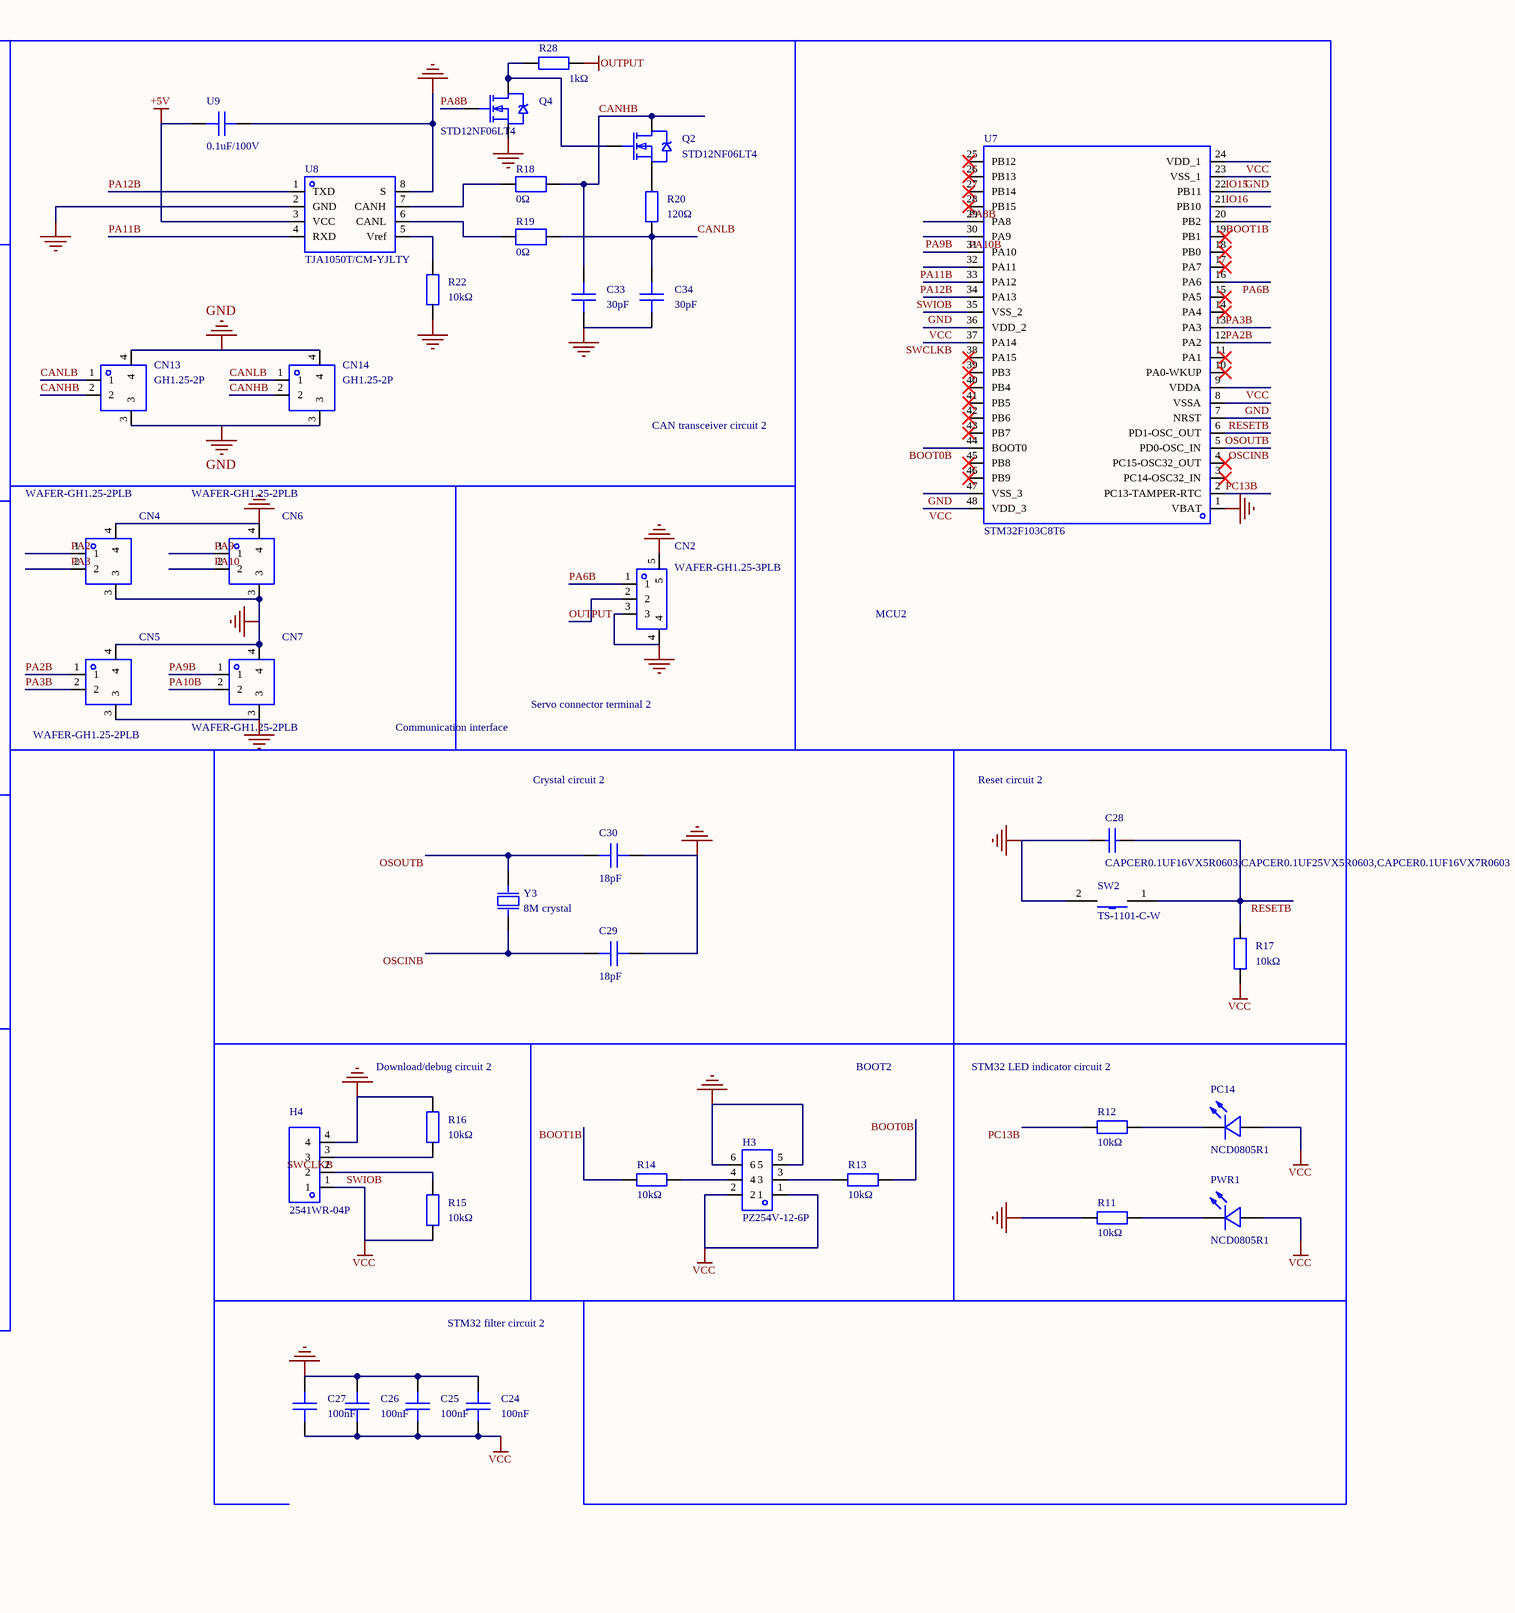
[diagram p0: MISC62500-4.schdoc, right]
# Altium project MISC62500-2.PrjPcb (part 2 of 2)
## Sheet MISC62500-4.schdoc (continued)
### Parts (continued)
Q2  STD12NF06LT4  [TO-252-3_L6.5-W5.8-P4.58-BL]
Q3  STD12NF06LT4  [TO-252-3_L6.5-W5.8-P4.58-BL]
Q4  STD12NF06LT4  [TO-252-3_L6.5-W5.8-P4.58-BL]
R1  10kΩ  [R0603]
R2  10kΩ  [R0603]
R3  10kΩ  [R0603]
R4  10kΩ  [R0603]
R5  10kΩ  [R0603]
R6  10kΩ  [R0603]
R7  10kΩ  [R0603]
R8  0Ω  [R0805]
R9  0Ω  [R0805]
R10  120Ω  [R0805]
R11  10kΩ  [R0603]
R12  10kΩ  [R0603]
R13  10kΩ  [R0603]
R14  10kΩ  [R0603]
R15  10kΩ  [R0603]
R16  10kΩ  [R0603]
R17  10kΩ  [R0603]
R18  0Ω  [R0805]
R19  0Ω  [R0805]
R20  120Ω  [R0805]
R21  10kΩ  [R0603]
R22  10kΩ  [R0603]
R27  1kΩ  [R0805]
R28  1kΩ  [R0805]
SW1  TS-1101-C-W  [SW-SMD_L6.0-W3.3-LS8.0]
SW2  TS-1101-C-W  [SW-SMD_L6.0-W3.3-LS8.0]
SW5  SK12D07VG4  [SW-TH_SK12D07VG4]
U1  STM32F103C8T6  [LQFP-48_L7.0-W7.0-P0.50-LS9.0-BL]
U2  0.1uF/100V  [C0805]
U3  AMS1117-5.0  [SOT-89-3_L4.5-W2.5-P1.50-LS4.2-BR]
U4  TJA1050T/CM-YJLTY  [SOIC-8_L4.9-W3.9-P1.27-LS6.0-BL]
U6  XT30U-F  [CONN-TH_XT30U-F]
U7  STM32F103C8T6  [LQFP-48_L7.0-W7.0-P0.50-LS9.0-BL]
U8  TJA1050T/CM-YJLTY  [SOIC-8_L4.9-W3.9-P1.27-LS6.0-BL]
U9  0.1uF/100V  [C0805]
Y2  8M crystal  [HC-49S_L11.5-W4.7-P4.88]
Y3  8M crystal  [HC-49S_L11.5-W4.7-P4.88]

### Blocks framed on the sheet
STM32 power circuit: C1-C4 LDO1
STM32 filter circuit: C5-C8
CAN transceiver circuit 2: C33 C34 CN13 CN14 Q2 Q4 R18-R20 R22 R28 U8 U9
MCU2: U7
STM32 LED indicator circuit: PC13 PWR R1 R2
Download/debug circuit: H2 R5 R6
Reset circuit: C9 R7 SW1
Communication interface: CN4-CN7
Servo connector terminal 2: CN2
Crystal circuit 2: C29 C30 Y3
Reset circuit 2: C28 R17 SW2
MCU: U1
Servo connector terminal: CN1
Voltage regulator module: C14-C17 U3
Download/debug circuit 2: H4 R15 R16
BOOT2: H3 R13 R14
STM32 LED indicator circuit 2: PC14 PWR1 R11 R12
CAN transceiver circuit: C18 C19 CN11 CN12 Q1 Q3 R8-R10 R21 R27 U2 U4

### Nets
+5V: C1.2 C2.2 C15.1 C17.1 LDO1.1(VIN) LDO1.3(CE) U2.1 U3.2(VOUT) U4.3(VCC) U8.3(VCC) U9.1
GND: C1.1 C2.1 C3.1 C4.1 C5.1 C6.1 C7.1 C8.1 C9.1 C10.2 C11.2 C14.1 C15.2 C16.1 C17.2 C18.1 C19.1 C24.1 C25.1 C26.1 C27.1 C28.1 C29.2 C30.2 C33.1 C34.1 CN1.3 CN1.4 CN1.5 CN2.3 CN2.4 CN2.5 CN3.1 CN3.2 CN4.3 CN4.4 CN5.3 CN5.4 CN6.3 CN6.4 CN7.3 CN7.4 CN10.1 CN10.2 CN11.3 CN11.4 CN12.3 CN12.4 CN13.3 CN13.4 CN14.3 CN14.4 H1.5 H1.6 H2.4 H3.5 H3.6 H4.4 LDO1.2(VSS) Q3.3(S) Q4.3(S) R1.2 R6.1 R11.2 R16.1 R21.1 R22.1 SW1.2 SW2.2 SW5.4 SW5.5 U1.1(VBAT) U1.8(VSSA) U1.23(VSS_1) U1.35(VSS_2) U1.47(VSS_3) U2.2 U3.1(ADJ/GND) U4.2(GND) U4.8(S) U6.1(-) U7.1(VBAT) U7.8(VSSA) U7.23(VSS_1) U7.35(VSS_2) U7.47(VSS_3) U8.2(GND) U8.8(S) U9.2
OUTPUT: C14.2 C16.2 CN1.2 CN2.2 R27.2 R28.2 SW5.2 U3.3(VIN)
VCC: C3.2 C4.2 C5.2 C6.2 C7.2 C8.2 C24.2 C25.2 C26.2 C27.2 H1.1 H1.2 H2.1 H3.1 H3.2 H4.1 LDO1.5(VOUT) PC13.1(+) PC14.1(+) PWR.1(+) PWR1.1(+) R5.2 R7.2 R15.2 R17.2 U1.9(VDDA) U1.24(VDD_1) U1.36(VDD_2) U1.48(VDD_3) U7.9(VDDA) U7.24(VDD_1) U7.36(VDD_2) U7.48(VDD_3)
BOOT0: R3.1 U1.44(BOOT0)
BOOT0B: R13.1 U7.44(BOOT0)
BOOT1: R4.2 U1.20(PB2)
BOOT1B: R14.2 U7.20(PB2)
CANH: C18.2 CN11.2 CN12.2 Q1.2(D) R8.2
CANHB: C33.2 CN13.2 CN14.2 Q2.2(D) R18.2
CANL: C19.2 CN11.1 CN12.1 R9.2 R10.1
CANLB: C34.2 CN13.1 CN14.1 R19.2 R20.1
IO4: U1.22(PB11)
IO5: U1.21(PB10)
IO15: U7.22(PB11)
IO16: U7.21(PB10)
OSCIN: C10.1 U1.5(PD0-OSC_IN) Y2.1(OSC1)
OSCINB: C29.1 U7.5(PD0-OSC_IN) Y3.1(OSC1)
OSOUT: C11.1 U1.6(PD1-OSC_OUT) Y2.2(OSC2)
OSOUTB: C30.1 U7.6(PD1-OSC_OUT) Y3.2(OSC2)
PA2: CN4.1 U1.12(PA2)
PA2B: CN5.1 U7.12(PA2)
PA3: CN4.2 U1.13(PA3)
PA3B: CN5.2 U7.13(PA3)
PA6: CN1.1 U1.16(PA6)
PA6B: CN2.1 U7.16(PA6)
PA8: Q3.1(G) U1.29(PA8)
PA8B: Q4.1(G) U7.29(PA8)
PA9: CN6.1 U1.30(PA9)
PA9B: CN7.1 U7.30(PA9)
PA10: CN6.2 U1.31(PA10)
PA10B: CN7.2 U7.31(PA10)
PA11: U1.32(PA11) U4.4(RXD)
PA11B: U7.32(PA11) U8.4(RXD)
PA12: U1.33(PA12) U4.1(TXD)
PA12B: U7.33(PA12) U8.1(TXD)
PC13: R2.2 U1.2(PC13-TAMPER-RTC)
PC13B: R12.2 U7.2(PC13-TAMPER-RTC)
POWER: SW5.1 U6.2(+)
RESET: C9.2 R7.1 SW1.1 U1.7(NRST)
RESETB: C28.2 R17.1 SW2.1 U7.7(NRST)
SWCLK: H2.3 R6.2 U1.37(PA14)
SWCLKB: H4.3 R16.2 U7.37(PA14)
SWIO: H2.2 R5.1 U1.34(PA13)
SWIOB: H4.2 R15.1 U7.34(PA13)
NetH1_3: H1.3 R3.2
NetH1_4: H1.4 R4.1
NetH3_3: H3.3 R13.2
NetH3_4: H3.4 R14.1
NetPC13_2: PC13.2(-) R2.1
NetPC14_2: PC14.2(-) R12.1
NetPWR1_2: PWR1.2(-) R11.1
NetPWR_2: PWR.2(-) R1.1
NetQ1_1: Q1.1(G) Q3.2(D) R27.1
NetQ1_3: Q1.3(S) R10.2
NetQ2_1: Q2.1(G) Q4.2(D) R28.1
NetQ2_3: Q2.3(S) R20.2
NetR8_1: R8.1 U4.7(CANH)
NetR9_1: R9.1 U4.6(CANL)
NetR18_1: R18.1 U8.7(CANH)
NetR19_1: R19.1 U8.6(CANL)
NetR21_2: R21.2 U4.5(Vref)
NetR22_2: R22.2 U8.5(Vref)

Not connected (* = marked no-connect by the designer): LDO1 4(NC)*; SW5 3*; U1 3(PC14-OSC32_IN)* 4(PC15-OSC32_OUT)* 10(PA0-WKUP)* 11(PA1)* 14(PA4)* 15(PA5)* 17(PA7)* 18(PB0)* 19(PB1)* 25(PB12)* 26(PB13)* 27(PB14)* 28(PB15)* 38(PA15)* 39(PB3)* 40(PB4)* 41(PB5)* 42(PB6)* 43(PB7)* 45(PB8)* 46(PB9)*; U7 3(PC14-OSC32_IN)* 4(PC15-OSC32_OUT)* 10(PA0-WKUP)* 11(PA1)* 14(PA4)* 15(PA5)* 17(PA7)* 18(PB0)* 19(PB1)* 25(PB12)* 26(PB13)* 27(PB14)* 28(PB15)* 38(PA15)* 39(PB3)* 40(PB4)* 41(PB5)* 42(PB6)* 43(PB7)* 45(PB8)* 46(PB9)*

### Notes on the sheet
- BOOT
- Crystal circuit
- (near SW5) Power switch
- STM32 filter circuit 2
- 2026-05-12
- Schematic
- Sheet
- Item code
- Reviewed
- Drawn
- Revision
- Size
- page
- Total
- A4
- 1
- 2

### Library data of the parts
C1 C4 C9 C28 = CAPCER0.1UF16VX5R0603,CAPCER0.1UF25VX5R0603,CAPCER0.1UF16VX7R0603: AddInBom: yes; ModelId: ac125912035d415993ca9572d50418b1; ModelName: C0603_L1.6-W0.8-H0.8; ModelTransform: 62.992,31.496,0,0,0,0,0,0,0; Symbol: CAPCER0.1UF16VX5R0603,CAPCER0.1UF25VX5R0603,CAPCER0.1UF16VX7R0603; Device: CAPCER0.1UF16VX5R0603,CAPCER0.1UF25VX5R0603,CAPCER0.1UF16VX7R0603; LCSC Part Name: CAPCER0.1UF16VX5R0603,CAPCER0.1UF25VX5R0603,CAPCER0.1UF16VX7R0603; SupplierPart: C9900012833; ManufacturerPart: CAPCER0.1UF16VX5R0603,CAPCER0.1UF25VX5R0603,CAPCER0.1UF16VX7R0603; Supplier Footprint: C0603; JLCPCB Part Class: Extended Part; Supplier: LCSC; ConvertToPcb: yes; FootprintName: C0603
C2 C3 = GRM188R71C105KE15D: Capacitance: 1uF; Tolerance: ±10%; Rated voltage: 16V; Dielectric (temp coefficient): X7R;; Manufacturer: muRata(村田); AddInBom: yes; ModelId: ac125912035d415993ca9572d50418b1; ModelName: C0603_L1.6-W0.8-H0.8; ModelTransform: 62.992,31.496,0,0,0,0,0,0,0; Symbol: GRM188R71C105KE15D; Device: GRM188R71C105KE15D; LCSC Part Name: 1uF ±10% 16V; SupplierPart: C77049; ManufacturerPart: GRM188R71C105KE15D; Supplier Footprint: 0603; JLCPCB Part Class: Extended Part; Datasheet: example.com/upload/public/pdf/source/20200305/C490387_23319AE8C154DEB24C505E6C82A8106A.pdf; Supplier: LCSC; ConvertToPcb: yes; FootprintName: C0603; Value: 1uF; Voltage Rated: 16V; Temperature Coefficient: X7R
C5-C8 C14 C15 C24-C27 = C1608X7S2A104K080AE: Capacitance: 100nF; Tolerance: ±10%; Rated voltage: 100V; Dielectric (temp coefficient): X7S;; Manufacturer: TDK; AddInBom: yes; ModelId: ac125912035d415993ca9572d50418b1; ModelName: C0603_L1.6-W0.8-H0.8; ModelTransform: 62.992,31.496,0,0,0,0,0,0,0; Symbol: C1608X7S2A104K080AE; Device: C1608X7S2A104K080AE; LCSC Part Name: 100nF ±10% 100V; SupplierPart: C3840667; ManufacturerPart: C1608X7S2A104K080AE; Supplier Footprint: 0603; JLCPCB Part Class: Extended Part; Datasheet: example.com/upload/public/pdf/source/20230606/B9E1D4FA5049A6C4984F2DC41D008D88.pdf; Supplier: LCSC; ConvertToPcb: yes; FootprintName: C0603; Value: 100nF; Voltage Rated: 100V; Temperature Coefficient: X7S
C10 C11 C29 C30 = C1608C0G1H180J080AA: Capacitance: 18pF; Tolerance: ±5%; Rated voltage: 50V; Dielectric (temp coefficient): C0G;; Manufacturer: TDK; AddInBom: yes; ModelId: ac125912035d415993ca9572d50418b1; ModelName: C0603_L1.6-W0.8-H0.8; ModelTransform: 62.992,31.496,0,0,0,0,0,0,0; Symbol: C1608C0G1H180J080AA; Device: C1608C0G1H180J080AA; LCSC Part Name: 18pF ±5% 50V; SupplierPart: C3902597; ManufacturerPart: C1608C0G1H180J080AA; Supplier Footprint: 0603; JLCPCB Part Class: Extended Part; Datasheet: example.com/upload/public/pdf/source/20230606/A83975C7E70EF5AFCD4A17254ABD78F2.pdf; Supplier: LCSC; ConvertToPcb: yes; FootprintName: C0603; Value: 18pF; Voltage Rated: 50V; Temperature Coefficient: C0G
C16 = CL10A106KP8NNNC: Capacitance: 10uF; Tolerance: ±10%; Rated voltage: 10V; Dielectric (temp coefficient): X5R;; Manufacturer: SAMSUNG(三星); AddInBom: yes; ModelId: ac125912035d415993ca9572d50418b1; ModelName: C0603_L1.6-W0.8-H0.8; ModelTransform: 62.992,31.496,0,0,0,0,0,0,0; Symbol: CL10A106KP8NNNC; Device: CL10A106KP8NNNC; LCSC Part Name: 10uF ±10% 10V; SupplierPart: C19702; ManufacturerPart: CL10A106KP8NNNC; Supplier Footprint: 0603; JLCPCB Part Class: Basic Part; Datasheet: example.com/upload/public/pdf/source/20160218/1457707763339.pdf; Supplier: LCSC; ConvertToPcb: yes; FootprintName: C0603; Value: 10uF; Voltage Rated: 10V; Temperature Coefficient: X5R
C17 = CL10A226MQ8NRNC: Capacitance: 22uF; Tolerance: ±20%; Rated voltage: 6.3V; Dielectric (temp coefficient): X5R;; Manufacturer: SAMSUNG(三星); AddInBom: yes; ModelId: ac125912035d415993ca9572d50418b1; ModelName: C0603_L1.6-W0.8-H0.8; ModelTransform: 62.992,31.496,0,0,0,0,0,0,0; Symbol: CL10A226MQ8NRNC; Device: CL10A226MQ8NRNC; LCSC Part Name: 22uF ±20% 6.3V; SupplierPart: C59461; ManufacturerPart: CL10A226MQ8NRNC; Supplier Footprint: 0603; JLCPCB Part Class: Basic Part; Datasheet: example.com/upload/public/pdf/source/20160218/1457707763339.pdf; Supplier: LCSC; ConvertToPcb: yes; FootprintName: C0603; Value: 22uF; Voltage Rated: 6.3V; Temperature Coefficient: X5R
C18 C19 C33 C34 = 0805N300J500CT: Capacitance: 30pF; Tolerance: ±5%; Rated voltage: 50V; Dielectric (temp coefficient): NP0;; Manufacturer: Walsin(华新科); AddInBom: yes; ModelId: 1ba041120af144c991958decab20d241; ModelName: C0805_L2.0-W1.3-H1.3; ModelTransform: 78.74,51.181,0,0,0,0,0,0.0005,0; Symbol: 0805N300J500CT; Device: 0805N300J500CT; LCSC Part Name: 30pF ±5% 50V; SupplierPart: C296096; ManufacturerPart: 0805N300J500CT; Supplier Footprint: 0805; JLCPCB Part Class: Extended Part; Datasheet: example.com/upload/public/pdf/source/20190509/C384834_C04286DA86A56A9914642D37A195BF18.pdf; Supplier: LCSC; ConvertToPcb: yes; FootprintName: C0805; Value: 30pF; Voltage Rated: 50V; Temperature Coefficient: NP0
CN1 CN2 = WAFER-GH1.25-3PLB: 插针结构:1x3P;间距:1.25mm;安装方式:立贴;参考系列:GH;总PIN数:3P;排数:1;每排PIN数:3;额定电流:1A;工作温度范围:-25℃~+85℃;; Manufacturer: XUNPU(讯普); AddInBom: yes; ModelId: 4873dadba1a240aabfda9d65a8d79f0f; ModelTransform: 277.9522,194.882,0,0,0,0,0,-21.89,0; Pins Structure: 1x3P; Pitch: 1.25mm; Reference Series: GH; Number of PINs Per Row: 3; Current Rating (Max): 1A; Symbol: WAFER-GH1.25-3PLB; Device: WAFER-GH1.25-3PLB; LCSC Part Name: 1x3P 间距:1.25mm 立贴 系列:GH; SupplierPart: C3029369; ManufacturerPart: WAFER-GH1.25-3PLB; Supplier Footprint: SMD,P=1.25mm; JLCPCB Part Class: Extended Part; Datasheet: example.com/upload/public/pdf/source/20220527/44F824AAC8C2B617205E15955FF9C23D.pdf; Supplier: LCSC; ConvertToPcb: yes; FootprintName: CONN-SMD_3P-P1.25_XUNPU_WAFER-GH1.25-3PLB; ModelName: CONN-SMD_3P-P1.25_XUNPU_WAFER-GH1.25-3PLB; Mounting Style: Vertical SMD; Number of Pins: 3P; Number of Rows: 1; Operating Temperature Range: -25℃~+85℃
CN3 CN10 = 2060-451/998-404: 结构:1x1P;间距:-;颜色:白色;安装方式:-;总PIN数:1P;每排PIN数:1;排数:1;额定电流:9A;额定电压:600V;线规 - AWG:18~24;线规 - 平方毫米:-;工作温度:-60℃~+105℃;; Manufacturer: WAGO(万可); AddInBom: yes; ModelId: 2b3842d5616144ad98afb9a8d8e70ac0; ModelTransform: 515.747,153.543,0,0,0,0,-20.512,0,0; Number of Positions or Pins: 1x1P; Number of PINs Per Row: 1; Current Rating: 9A; Voltage Rating (Max): 600V; Wire Gauge - AWG: 18~24; Symbol: 2060-451/998-404; Device: 2060-451/998-404; LCSC Part Name: 1x1P 每排P数:1 排数:1; SupplierPart: C2765054; ManufacturerPart: 2060-451/998-404; Supplier Footprint: SMD,P=4mm; JLCPCB Part Class: Extended Part; Datasheet: example.com/upload/public/pdf/source/20210406/C2765054_9C4366D01569C61DE4D9DE6FC53C47DE.pdf; Supplier: LCSC; ConvertToPcb: yes; FootprintName: CONN-SMD_L12.7-W3.9_2060-451-998-404; ModelName: CONN-SMD_L12.7-W3.9_2060-451-998-404; Pitch: -; Color: White; Mounting Type: -; Number of Pins: 1P; Number of Rows: 1; Wire Gauge - mm2: -; Operating Temperature: -60℃~+105℃
CN4-CN7 CN11-CN14 = WAFER-GH1.25-2PLB: 插针结构:1x2P;间距:1.25mm;安装方式:立贴;参考系列:GH;总PIN数:2P;排数:1;每排PIN数:2;行距:-;额定电流:1A;触头材质:黄铜;触头镀层:-;工作温度范围:-25℃~+85℃;; Manufacturer: XUNPU(讯普); AddInBom: yes; ModelId: 0c15e313285a4ca08f633459465ca938; ModelTransform: 226.7712,194.8815,0,180,0,0,0,-11.968,0; Pins Structure: 1x2P; Pitch: 1.25mm; Reference Series: GH; Number of PINs Per Row: 2; Current Rating: 1A; Voltage Rating: 125V; Plastic Material: LCP; Supplementary Features: Auxiliary solder pad; Z-Height of the Board: 4.2mm; X-Length of Bottom Edge on Board (Spacing Line): 5.75mm; Y-Width of Bottom Edge on Board: 4.95mm; Symbol: WAFER-GH1.25-2PLB; Device: WAFER-GH1.25-2PLB; LCSC Part Name: 1x2P 间距:1.25mm 立贴 系列:GH; SupplierPart: C3029368; Supplier Footprint: SMD,P=1.25mm; JLCPCB Part Class: Extended Part; Datasheet: example.com/upload/public/pdf/source/20220527/44F824AAC8C2B617205E15955FF9C23D.pdf; Supplier: LCSC; ConvertToPcb: yes; FootprintName: CONN-TH_2P-P1.25_XUNPU_WAFER-GH1.25-2PLB; ModelName: CONN-TH_2P-P1.25_XUNPU_WAFER-GH1.25-2PLB; Mounting Type: Vertical SMD; Number of Pins: 2P; Number of Rows: 1; Row Spacing: -; Contact Material: Brass; Contact Plating: -; Operating Temperature: -25℃~+85℃; Flame Retardant Rating: -; Color: Beige
  CN4-CN7: ManufacturerPart: WAFER-GH1.25-2PLB
  CN11-CN14: Manufacturer Part: GH1.25-2P
H1 H3 = PZ254V-12-6P: 插针结构:2x3P;间距:2.54mm;行距:2.54mm;圆针/方针:方针;安装类型:直插;排数:双排;总PIN位数:6P;额定电流:-;额定电压:-;配合针长度:6mm;塑高:2.5mm;端接针长度:3mm;触头材质:黄铜;触头镀层:-;工作温度范围:-40℃~+105℃;颜色:黑色;; Manufacturer: XFCN(兴飞); AddInBom: yes; ModelId: 6bc2347a11144808b30843246bd74e32; ModelTransform: 299.9994,200,0,0,0,0,0,0,-118.11; Pin Structure: 2x3P; Pitch: 2.54mm; Circluar Pins/Square Pins: Square pin; Symbol: PZ254V-12-6P; Device: PZ254V-12-6P; LCSC Part Name: 间距:2.54mm 2x3P 直插 方针; SupplierPart: C492420; ManufacturerPart: PZ254V-12-6P; Supplier Footprint: 插件,P=2.54mm; JLCPCB Part Class: Extended Part; Datasheet: example.com/upload/public/pdf/source/20200309/C492420_BAECB307B001054C09D200388220EAE6.pdf; Supplier: LCSC; ConvertToPcb: yes; FootprintName: HDR-TH_6P-P2.54-V-M-R2-C3-S2.54; ModelName: HDR-TH_6P-P2.54-V-M-R2-C3-S2.54; Row Spacing: 2.54mm; Mounting Type: Through-hole; Number of Rows: Dual row; Number of Pins: 6P; Current Rating (Max): -; Voltage Rating (Max): -; Length of Mating Pin: 6mm; Insulation Height: 2.5mm; Length of End Connection Pin: 3mm; Contact Material: Brass; Contact Plating: -; Operating Temperature Range: -40℃~+105℃; Color: Black
H2 H4 = 2541WR-04P: Pitch: 2.54mm; Mounting: right-angle THT; Rows: single; Mating pin length: 6mm; Plastic height: 2.54mm;; Manufacturer: HanElectricity(瀚源); AddInBom: yes; ModelId: 91498ce4cc554a519d8986aa62dd6bb1; ModelTransform: 399.999,405.511,0,0,0,0,0,-188.976,-118.11; Symbol: 2541WR-04P; Device: 2541WR-04P; LCSC Part Name: 间距:2.54mm 弯插; SupplierPart: C5383097; ManufacturerPart: 2541WR-04P; Supplier Footprint: 弯插,P=2.54mm; JLCPCB Part Class: Extended Part; Datasheet: example.com/upload/public/pdf/source/20230410/E05CF6F056E300DA9C417F17E461DF93.pdf; Supplier: LCSC; ConvertToPcb: yes; FootprintName: HDR-TH_4P-P2.54-H-M-W10.4-N; ModelName: HDR-TH_4P-P2.54-H-M-W10.4-N; Mounting Type: Right-angle THT; Number of Rows: Single row; Length of Mating Pin: 6mm; Insulation Height: 2.54mm
LDO1 = ME6211C33M5G-N: Output type: fixed; Max input voltage: 6V; Output voltage: 3.3V; Max output current: 500mA; PSRR: 70dB; Output polarity: positive;; Manufacturer: MICRONE(南京微盟); AddInBom: yes; ModelId: 0a2a1b8f50944f73965918ad6e5fe167; ModelName: SOT-23-5_L2.9-W1.6-H1.1-LS2.8-P0.95; ModelTransform: 118.60433,114.173,0,90,0,0,0.0005,0.0005,0; Dropout Voltage: 260mV@(200mA); Number of Outputs: 1; Symbol: ME6211C33M5G-N; Device: ME6211C33M5G-N; LCSC Part Name: 输入6V 输出3.3V 500mA; SupplierPart: C82942; ManufacturerPart: ME6211C33M5G-N; Supplier Footprint: SOT-23-5; JLCPCB Part Class: Extended Part; Datasheet: example.com/upload/public/pdf/source/20170918/C82942_1505727073070976520.pdf; Supplier: LCSC; ConvertToPcb: yes; FootprintName: SOT-23-5_L3.0-W1.7-P0.95-LS2.8-BL; Output Type: Fixed; Maximum Input Voltage: 6V; Output Voltage: 3.3V; MAX Output Current: 500mA; Power Supply Rejection Ratio (PSRR): 70dB; Output Polarity: Positive
PC13 PC14 PWR PWR1 = NCD0805R1: 灯头类型:-;发光颜色:红色;正向电压(VF):1.6V~2.6V;功率:65mW;正向电流:20mA;主波长:615nm~630nm;二极管配置:独立二极管;透镜颜色:无色透明透镜;色温:-;发光强度:67mcd~195mcd;发光角度:130°;载带方式:-;工作温度:-30℃~+85℃;; Manufacturer: 国星光电; Symbol: FC-2012HRK-620D; AddInBom: yes; ModelId: 6ccd75a2b5134d6ab756ecf3c14a7290; ModelName: LED0805-RD; ModelTransform: 79.527,49.2125,0,0,0,0,0,0,0; Emitted Color: Red; Power Dissipation: 65mW; Forward Current: 20mA; Diode Configuration: Single diode; Lens Color: Clear lens; Viewing Angle: 130°; Device: NCD0805R1; LCSC Part Name: NCD0805R1; SupplierPart: C84256; ManufacturerPart: NCD0805R1; Supplier Footprint: 0805; JLCPCB Part Class: Basic Part; Datasheet: example.com/upload/public/pdf/source/20200820/C84256_F0A75A43B3EAD75808600A0514C76B99.pdf; Supplier: LCSC; ConvertToPcb: yes; FootprintName: LED0805-R-RD; Lamp Holder Type: -; Forward Voltage (VF): 1.6V~2.6V; Dominant Wavelength: 615nm~630nm; Peak Wavelength: -; Color Temperature: -; Luminous Intensity: 67mcd~195mcd; Mounting Sytle: -; Operating Temperature: -30℃~+85℃
Q1-Q4 = STD12NF06LT4: 类型:1个N沟道;漏源电压(Vdss):60V;连续漏极电流(Id):12A;导通电阻(RDS(on)@Vgs,Id):100mΩ@10V,6A;功率(Pd):42.8W;阈值电压(Vgs(th)@Id):2V@250uA;; Manufacturer: ST(意法半导体); AddInBom: yes; ModelId: b30bfce30d0f4a429b5e4d5ada8cad65; ModelTransform: 249.9995,380.57715,0,0,0,0,-0.118,24.409,0; Type: 1 N-channel; Drain Source Voltage (Vdss): 60V; Continuous Drain Current (Id): 12A; Power Dissipation (Pd): 42.8W; Symbol: STD12NF06LT4; Device: STD12NF06LT4; LCSC Part Name: 1个N沟道 耐压:60V 电流:12A; SupplierPart: C92516; ManufacturerPart: STD12NF06LT4; Supplier Footprint: TO-252-2(DPAK); JLCPCB Part Class: Extended library; Datasheet: example.com/upload/public/pdf/source/20161229/1482979427929.pdf; Supplier: LCSC; ConvertToPcb: yes; FootprintName: TO-252-3_L6.5-W5.8-P4.58-BL; ModelName: TO-252-3_L6.5-W5.8-P4.58-BL; Drain Source On Resistance (RDS(on)@Vgs,Id): 100mΩ@10V,6A; Gate Threshold Voltage (Vgs(th)@Id): 2V@250uA
R1-R7 R11-R17 R21 R22 = ACD03K1002FT: Resistor type: thick film resistor; Resistance: 10kΩ; Tolerance: ±1%; Power: 100mW; Max working voltage: 50V; Temp coefficient: ±100ppm/℃;; Manufacturer: FH(风华); AddInBom: yes; ModelId: fc143cca1e79419f9cd78b61e9279f08; ModelTransform: 31.8897,63.7794,0,90,0,0,0,0,0; Symbol: ACD03K1002FT; Device: ACD03K1002FT; LCSC Part Name: 厚膜电阻 10kΩ ±1% 100mW; SupplierPart: C347053; ManufacturerPart: ACD03K1002FT; Supplier Footprint: 0603; JLCPCB Part Class: Extended Part; Datasheet: example.com/upload/public/pdf/source/20181211/C347075_B548F78FC3FAB5F0A0CE430650CC5FDF.pdf; Supplier: LCSC; ConvertToPcb: yes; FootprintName: R0603; ModelName: R0603; Type: Thick film resistor; Value: 10kΩ; Power(Watts): 100mW; Overload Voltage (Max): 50V; Temperature Coefficient: ±100ppm/℃; Operating Temperature Range: -55℃~+155℃
R8 R9 R18 R19 = RHC-05000FT: Resistor type: thick film resistor; Resistance: 0Ω; Tolerance: ±1%;; Manufacturer: FH(风华); AddInBom: yes; ModelId: 37a81e68749a4138bd2dfa6897b24b85; ModelName: R0805_L2.0-W1.3-H0.6; ModelTransform: 78.74,51.181,0,0,0,0,0,-0.0005,0; Symbol: RHC-05000FT; Device: RHC-05000FT; LCSC Part Name: 厚膜电阻 0Ω ±1%; SupplierPart: C880283; ManufacturerPart: RHC-05000FT; Supplier Footprint: 0805; JLCPCB Part Class: Extended Part; Datasheet: example.com/upload/public/pdf/source/20201103/C880283_DE5575B69A2A5077A879474FF10E0F68.pdf; Supplier: LCSC; ConvertToPcb: yes; FootprintName: R0805; Type: Thick film resistor; Value: 0Ω; Tolerance: ±1%
R10 R20 = TC0525F1200T5E: Resistor type: thin film resistor; Resistance: 120Ω; Tolerance: ±1%; Power: 250mW; Max working voltage: 150V; Temp coefficient: ±25ppm/℃;; Manufacturer: UNI-ROYAL(厚声); AddInBom: yes; ModelId: 37a81e68749a4138bd2dfa6897b24b85; ModelName: R0805_L2.0-W1.3-H0.6; ModelTransform: 78.74,51.181,0,0,0,0,0,-0.0005,0; Symbol: TC0525F1200T5E; Device: TC0525F1200T5E; LCSC Part Name: 120Ω ±1% 250mW 薄膜电阻; SupplierPart: C61683; ManufacturerPart: TC0525F1200T5E; Supplier Footprint: 0805; JLCPCB Part Class: Extended Part; Datasheet: example.com/upload/public/pdf/source/20190904/C425668_F2F639A313B6F33D501F342892FD5229.pdf; Supplier: LCSC; ConvertToPcb: yes; FootprintName: R0805; Type: Thin film resistor; Value: 120Ω; Power(Watts): 250mW; Overload Voltage (Max): 150V; Temperature Coefficient: ±25ppm/℃; Operating Temperature Range: -55℃~+155℃
R27 R28 = 0805W8F1001T5E: Resistor type: thick film resistor; Resistance: 1kΩ; Tolerance: ±1%; Power: 125mW; Max working voltage: 150V; Temp coefficient: ±100ppm/℃;; Manufacturer: UNI-ROYAL(厚声); AddInBom: yes; ModelId: 37a81e68749a4138bd2dfa6897b24b85; ModelName: R0805_L2.0-W1.3-H0.6; ModelTransform: 78.74,51.181,0,0,0,0,0,-0.0005,0; Symbol: 0805W8F1001T5E; Device: 0805W8F1001T5E; LCSC Part Name: 1kΩ ±1% 125mW 厚膜电阻; SupplierPart: C17513; ManufacturerPart: 0805W8F1001T5E; Supplier Footprint: 0805; JLCPCB Part Class: Basic Part; Datasheet: example.com/upload/public/pdf/source/20200306/C422600_1E6D84923E4A46A82E41ADD87F860B5C.pdf; Supplier: LCSC; ConvertToPcb: yes; FootprintName: R0805; Type: Thick film resistor; Value: 1kΩ; Power(Watts): 125mW; Overload Voltage (Max): 150V; Temperature Coefficient: ±100ppm/℃; Operating Temperature Range: -55℃~+155℃
SW1 SW2 = TS-1101-C-W: 电路结构:单刀单掷;按钮形状:矩形按钮;作用力:260gf;安装方式:立贴;开关长度:6mm;开关宽度:3.6mm;开关高度:2.5mm;带支架:不带;触点电流:50mA;额定电压(AC):-;额定电压(DC):12V;额定功率:-;绝缘电阻:-;带灯:无;机械寿命:5万次;; Manufacturer: XKB Connectivity(中国星坤); AddInBom: yes; ModelId: b2f4ea9f0afc4b0786d53dba66ceb9e4; ModelName: SW-SMD_L6.0-W3.3-H5-LS8.0; ModelTransform: 314.96,129.921,0,0,0,0,0,0,0; Circuit: SPST; Actuator Style: Rectangular button; Operating Force: 260gf; Switch Length: 6mm; Switch Width: 3.6mm; Switch Height: 2.5mm; Strike Gundam: Without; Contact Current: 50mA; Voltage Rating (DC): 12V; Actuator/Cap Color: White with light green; With Lamp: None; Mechanical Life: 5 x 10k cycles; Symbol: TS-1101-C-W; Device: TS-1101-C-W; LCSC Part Name: 6*3.6*2.5mm 立贴 轻触开关; SupplierPart: C318938; ManufacturerPart: TS-1101-C-W; Supplier Footprint: SMD; JLCPCB Part Class: Extended Part; Datasheet: example.com/upload/public/pdf/source/20200227/C318938_C2E53B1EEDE37D980A33616AC086DE53.pdf; Supplier: LCSC; ConvertToPcb: yes; FootprintName: SW-SMD_L6.0-W3.3-LS8.0; Mounting Style: Vertical SMD; Voltage Rating (AC): -; Power Rating: -; Insulation Resistance: -; IP Rating: -; Pin Style: -; Operating Temperature: -30℃~+85℃
SW5 = SK12D07VG4: 电路结构:单刀双掷;安装方式:-;额定电流(DC):500mA;额定电压(DC):50V;额定电流(AC):-;额定电压(AC):-;机械寿命:5千次;; Manufacturer: SHOU HAN(首韩); AddInBom: yes; ModelId: 773c51563d484e3a80810244c5d56a16; ModelName: SW-TH_L8.7-W4.4-H4.0-P2.0; ModelTransform: 338.582,279.527,0,0,0,0,0,-51.181,-125.984; Circuit: SPDT; Actuator Style: Rectangular post; Pin Style: PC pin; Switch Height: 8.8mm; Current Rating (DC): 500mA; Voltage Rating (DC): 50V; Mechanical Life: 5 x 1k cycles; Symbol: SK12D07VG4; Device: SK12D07VG4; LCSC Part Name: 3脚2档位 卧插 滑动开关; SupplierPart: C393937; ManufacturerPart: SK12D07VG4; Supplier Footprint: 插件; JLCPCB Part Class: Extended library; Datasheet: example.com/upload/public/pdf/source/20190521/C393937_939FE26E571CC67D2D532E953108A1B0.pdf; Supplier: LCSC; ConvertToPcb: yes; FootprintName: SW-TH_SK12D07VG4; Mounting Style: -; Current Rating (AC): -; Voltage Rating (AC): -; Operating Temperature: -
U1 U7 = STM32F103C8T6: CPU core: ARM-M3; Max CPU frequency: 72MHz; Application: -;; Manufacturer: ST(意法半导体); AddInBom: yes; ModelId: 093be70396ff421eb2cdb946d5311efc; ModelName: LQFP-48_L7.0-W7.0-H1.4-LS9.0-P0.50; ModelTransform: 354.331,354.331,0,0,0,0,0,0,0; Program Storage Size: 64KB; Program Memory Type: FLASH; GPIO Ports Number: 37; ADC (Bit): 12bit; Low Voltage Detection Threshold: 2V~3.6V; Symbol: STM32F103C8T6; Device: STM32F103C8T6; LCSC Part Name: 主流增强型ARM Cortex-M3 MCU，具有64 KB Flash、72 MHz CPU、电机控制、USB和CAN; SupplierPart: C8734; ManufacturerPart: STM32F103C8T6; Supplier Footprint: LQFP-48(7x7); JLCPCB Part Class: Extended library; Datasheet: example.com/upload/public/pdf/source/20220812/8363ACEC51AD55ECEB84799464F7CB85.pdf; Supplier: LCSC; ConvertToPcb: yes; FootprintName: LQFP-48_L7.0-W7.0-P0.50-LS9.0-BL; CPU Core: ARM-M3; CPU Maximum Speed: 72MHz; Application Area: -
U2 U9 = 0.1uF/100V_C9900010259: AddInBom: yes; ModelId: 1ba041120af144c991958decab20d241; ModelName: C0805_L2.0-W1.3-H1.3; ModelTransform: 78.74,51.181,0,0,0,0,0,0.0005,0; Symbol: 0.1UF/100V; Device: 0.1uF/100V_C9900010259; LCSC Part Name: 0.1uF/100V; SupplierPart: C9900010259; ManufacturerPart: 0.1uF/100V; Supplier Footprint: C0805; JLCPCB Part Class: Extended Part; Supplier: LCSC; ConvertToPcb: yes; FootprintName: C0805
U3 = AMS1117-5.0: Output type: fixed; Max input voltage: 18V; Output voltage: 5V; Output current: 1A; PSRR: 70dB@(120Hz); Output polarity: positive;; Manufacturer: Slkor(萨科微); Symbol: AMS1117-5.0_C880753; AddInBom: yes; ModelId: 6db690b7897d4d18a30d90c1b89525ee; ModelName: SOT-89-3_L4.3-W2.5-H1.6-LS4.1-P1.50; ModelTransform: 161.417,169.291,0,180,0,0,-11.808,0,0; Number of Outputs: 1; Device: AMS1117-5.0; LCSC Part Name: AMS1117-5.0; SupplierPart: C880753; ManufacturerPart: AMS1117-5.0; Supplier Footprint: SOT-89-3; JLCPCB Part Class: Extended library; Datasheet: example.com/upload/public/pdf/source/20190906/C426566_95BE246DE70C248781207323626ADB09.pdf; Supplier: LCSC; ConvertToPcb: yes; FootprintName: SOT-89-3_L4.5-W2.5-P1.50-LS4.2-BR; Output Type: Fixed; Maximum Input Voltage: 18V; Output Voltage: 5V; Output Current: 1A; Power Supply Rejection Ratio (PSRR): 70dB@(120Hz); Feature: Thermal protection (TSD); Operating Temperature: -40℃~+125℃@(Tj); Output Polarity: Positive
U4 U8 = TJA1050T/CM-YJLTY: AddInBom: yes; ModelId: e81d2f7d937b4a6ab1dca543ff5d56a4; ModelName: SOIC-8_L4.9-W3.9-H1.7-LS6.0-P1.27; ModelTransform: 189.751,236.22,0,0,0,0,0.0005,0.0005,0; Symbol: TJA1050T/CM-YJLTY; Device: TJA1050T/CM-YJLTY; LCSC Part Name: TJA1050T/CM-YJLTY; SupplierPart: C2911428; ManufacturerPart: TJA1050T/CM-YJLTY; Supplier Footprint: SOIC-8; JLCPCB Part Class: Extended Part; Supplier: LCSC; ConvertToPcb: yes; FootprintName: SOIC-8_L4.9-W3.9-P1.27-LS6.0-BL
U6 = XT30U-F: Category: -; Type 1: -;; Manufacturer: AMASS(艾迈斯); AddInBom: yes; ModelId: e15dd3b23be94d50b949f17926224bae; ModelTransform: 401.574,205.1177,0,0,0,0,-0.001,0.003,-118.11; Brand: ams; InterfaceType: Female; Symbol: XT30U-F; Device: XT30U-F; LCSC Part Name: AMASS(艾迈斯)轻量版锂电池插头母头 XT30U-F; SupplierPart: C99102; ManufacturerPart: XT30U-F; Supplier Footprint: -; JLCPCB Part Class: Extended library; Datasheet: example.com/upload/public/pdf/source/20190916/C428721_B0ECB8C5937139CEFE8736D2D3175B0E.pdf; Supplier: LCSC; ConvertToPcb: yes; FootprintName: CONN-TH_XT30U-F; ModelName: CONN-TH_XT30U-F; Model: XT30U-F; Power: -; Output: -; Input: -; Size: -; Interface: -; Type: Plug; Colour: Yellow; MaximumCurrent: -; RatedVoltage: -; Type1: -; NumberOfUSBHoles: -; MetalMaterial: -; InsulationMaterial: -; RatedCurrent: -; RecommendedWireGauge: -; FlameRetardantGrade: -; contact resistance: -; Belt length: -; specifications: -
Y2 Y3 = 8M晶振_C9900011272: ManufacturerPart: 8M晶振; Device: 8M crystal_C9900011272; AddInBom: yes; ModelId: 8681f9edbc4c49baa7439b9863851e5c; ModelTransform: 452.755,183.4642,0,0,0,0,0,0,-137.795; Symbol: 8M crystal; LCSC Part Name: 8M晶振; SupplierPart: C9900011272; Supplier Footprint: HC-49S; JLCPCB Part Class: Extended Part; Supplier: LCSC; ConvertToPcb: yes; FootprintName: HC-49S_L11.5-W4.7-P4.88; ModelName: HC-49S_L11.5-W4.7-P4.88

## Nets that join several sheets
+5V: MISC62500-3 (6 pins), MISC62500-4 (11 pins)
GND: MISC62500-3 (25 pins), MISC62500-4 (89 pins)
VCC: MISC62500-3 (10 pins), MISC62500-4 (33 pins)
IO4: MISC62500-3 (U14.4), MISC62500-4 (U1.22)
IO5: MISC62500-3 (U14.5), MISC62500-4 (U1.21)
IO15: MISC62500-3 (U14.8), MISC62500-4 (U7.22)
IO16: MISC62500-3 (U14.9), MISC62500-4 (U7.21)